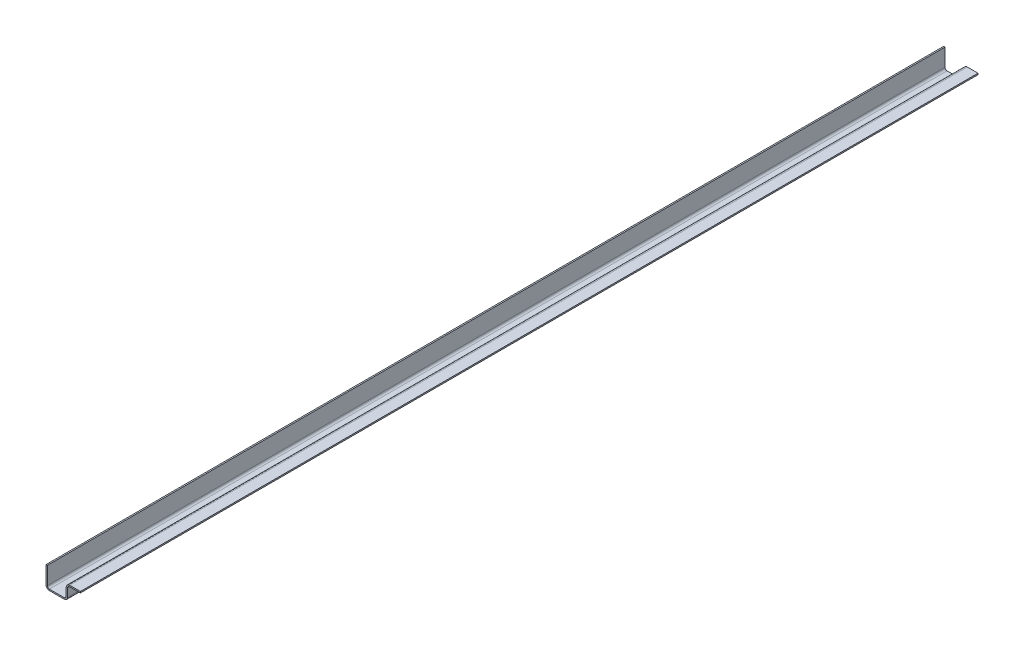
from build123d import *

# Parameters (mm, degrees)
EXTRUDE_1_DEPTH = 665.5


with BuildPart() as part:
    # 草图1 → 拉伸-薄壁1 (new, symmetric)
    with BuildSketch(Plane.XY):
        with BuildLine():
            Line((-1, 30), (-1, 4))
            ThreePointArc((-1, 4), (0.464466094, 0.464466094), (4, -1))
            Line((4, -1), (26, -1))
            ThreePointArc((26, -1), (29.535533906, 0.464466094), (31, 4))
            Line((31, 4), (31, 16))
            ThreePointArc((31, 16), (31.878679656, 18.121320344), (34, 19))
            Line((34, 19), (50, 19))
            Line((50, 19), (50, 21))
            Line((50, 21), (34, 21))
            ThreePointArc((34, 21), (30.464466094, 19.535533906), (29, 16))
            Line((29, 16), (29, 4))
            ThreePointArc((29, 4), (28.121320344, 1.878679656), (26, 1))
            Line((26, 1), (4, 1))
            ThreePointArc((4, 1), (1.878679656, 1.878679656), (1, 4))
            Line((1, 4), (1, 30))
            Line((1, 30), (-1, 30))
        make_face()
    extrude(amount=EXTRUDE_1_DEPTH, both=True)


solid = part.part
